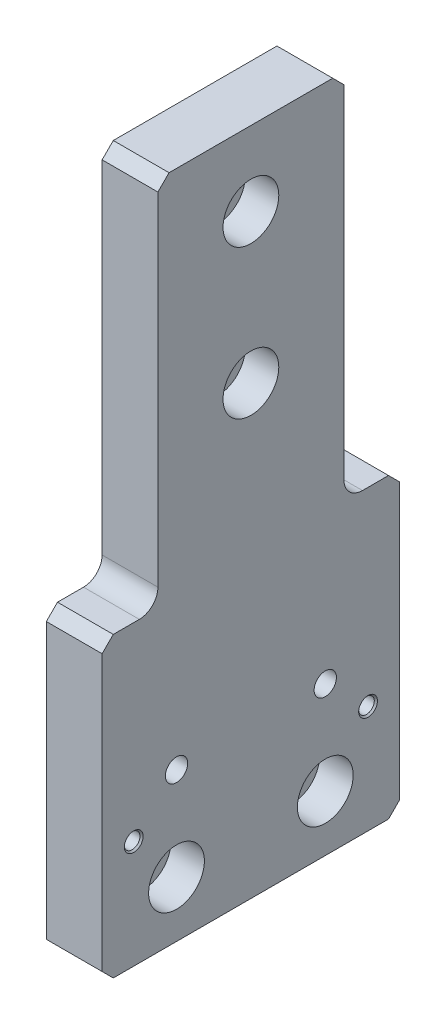
from build123d import *

# Parameters (mm, degrees)
BOSS_EXTRUDE1_DEPTH                                  = 15
M5_TAPPED_HOLE1_D                                    = 4.2
M5_TAPPED_HOLE1_DEPTH                                = 12.4
M5_TAPPED_HOLE1_CSINK_D                              = 5.05
M5_TAPPED_HOLE1_CSINK_ANGLE                          = 90
M5_TAPPED_HOLE1_TIP                                  = 1.2618073
CBORE_FOR_M8_HEXAGON_SOCKET_HEAD_CAP_SCR_D           = 9
CBORE_FOR_M8_HEXAGON_SOCKET_HEAD_CAP_SCR_CBORE_D     = 15
CBORE_FOR_M8_HEXAGON_SOCKET_HEAD_CAP_SCR_CBORE_DEPTH = 9
CBORE_FOR_M8_HEXAGON_SOCKET_HEAD_CAP_2_D             = 9
CBORE_FOR_M8_HEXAGON_SOCKET_HEAD_CAP_2_CBORE_D       = 15
CBORE_FOR_M8_HEXAGON_SOCKET_HEAD_CAP_2_CBORE_DEPTH   = 9
F_6_0MM_BLIND_HOLE_1_D                               = 6
FILLET1_R                                            = 5
CHAMFER1_SIZE                                        = 3


with BuildPart() as part:
    # Sketch1 → Boss-Extrude1 (new body)
    with BuildSketch(Plane(origin=(0, 0, 0), x_dir=(0, 0, -1), z_dir=(1, 0, 0))):
        Polygon((40, 0), (-40, 0), (-40, 80), (-25, 80), (-25, 180), (25, 180), (25, 80), (40, 80), align=None)
    extrude(amount=BOSS_EXTRUDE1_DEPTH)

    # M5 Tapped Hole1
    with Locations(Plane(origin=(15, 0, 0), x_dir=(0, 0, -1), z_dir=(1, 0, 0))):
        with Locations((31.5, 29), (-31.5, 29)):
            CounterSinkHole(M5_TAPPED_HOLE1_D / 2, M5_TAPPED_HOLE1_CSINK_D / 2, depth=M5_TAPPED_HOLE1_DEPTH, counter_sink_angle=M5_TAPPED_HOLE1_CSINK_ANGLE)
            with Locations((0, 0, -(M5_TAPPED_HOLE1_DEPTH + M5_TAPPED_HOLE1_TIP / 2))):  # 118° drill point
                Cone(0, M5_TAPPED_HOLE1_D / 2, M5_TAPPED_HOLE1_TIP, mode=Mode.SUBTRACT)

    # CBORE for M8 Hexagon socket head cap scr (through all)
    with Locations(Plane(origin=(15, 0, 0), x_dir=(0, 0, -1), z_dir=(1, 0, 0))):
        with Locations((0, 160), (0, 120)):
            CounterBoreHole(CBORE_FOR_M8_HEXAGON_SOCKET_HEAD_CAP_SCR_D / 2, CBORE_FOR_M8_HEXAGON_SOCKET_HEAD_CAP_SCR_CBORE_D / 2, CBORE_FOR_M8_HEXAGON_SOCKET_HEAD_CAP_SCR_CBORE_DEPTH)

    # CBORE for M8 Hexagon socket head cap 2 (through all)
    with Locations(Plane(origin=(15, 0, 0), x_dir=(0, 0, -1), z_dir=(1, 0, 0))):
        with Locations((-20, 15), (20, 15)):
            CounterBoreHole(CBORE_FOR_M8_HEXAGON_SOCKET_HEAD_CAP_2_D / 2, CBORE_FOR_M8_HEXAGON_SOCKET_HEAD_CAP_2_CBORE_D / 2, CBORE_FOR_M8_HEXAGON_SOCKET_HEAD_CAP_2_CBORE_DEPTH)

    # Ø6.0mm blind hole 1 (through all)
    with Locations(Plane(origin=(15, 0, 0), x_dir=(0, 0, -1), z_dir=(1, 0, 0))):
        with Locations((-20, 40), (20, 40)):
            Hole(F_6_0MM_BLIND_HOLE_1_D / 2)

    # Fillet1
    fillet1_edges = [part.edges().sort_by_distance(p)[0] for p in [
        (7.5, 80, 25),
        (7.5, 80, -25),
    ]]
    fillet(fillet1_edges, radius=FILLET1_R)

    # Chamfer1
    chamfer1_edges = [part.edges().sort_by_distance(p)[0] for p in [
        (7.5, 180, 25),
        (7.5, 180, -25),
        (7.5, 80, -40),
        (7.5, 0, -40),
        (7.5, 0, 40),
        (7.5, 80, 40),
    ]]
    chamfer(chamfer1_edges, length=CHAMFER1_SIZE)


solid = part.part
